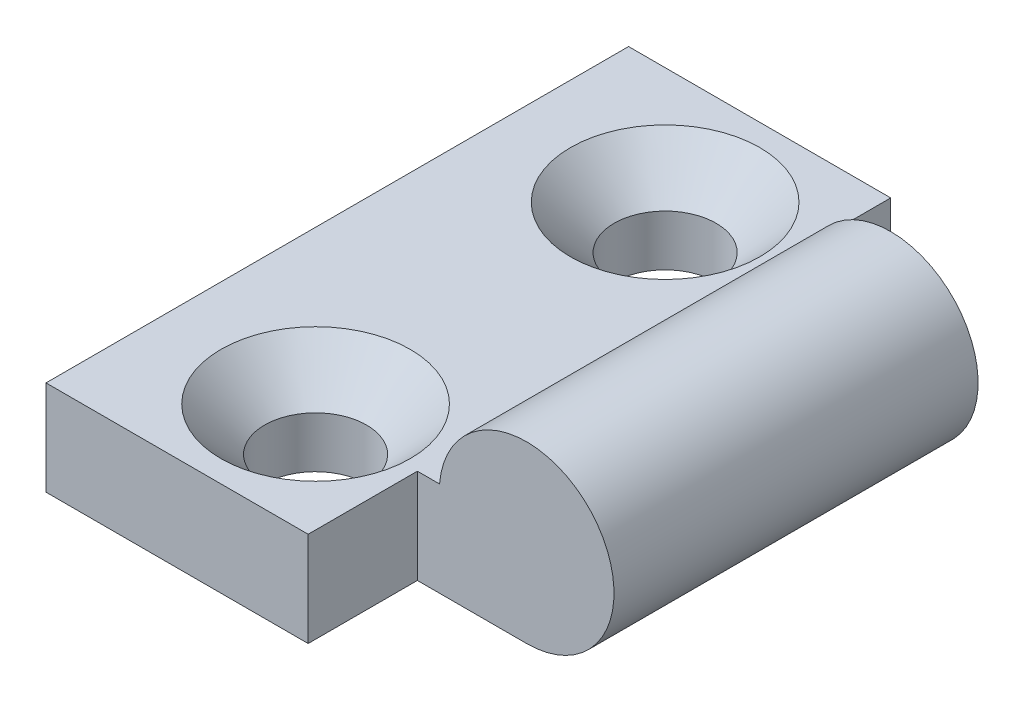
from build123d import *

# Parameters (mm, degrees)
SKETCH_1_W          = 25.5
SKETCH_1_H          = 40
EXTRUDE_1_DEPTH     = 6.5
SKETCH_2_R          = 6
EXTRUDE_2_DEPTH     = 40
SKETCH_3_W          = 13.5
SKETCH_3_H          = 7.5
CUT_EXTRUDE_1_DEPTH = 30.925950277
SKETCH_5_R          = 3.5
CUT_EXTRUDE_2_DEPTH = 29.174678348
CHAMFER_1_SIZE      = 3


with BuildPart() as part:
    # 草图1 → 凸台-拉伸1 (new body)
    with BuildSketch(Plane(origin=(0, 0, 0), x_dir=(1, 0, 0), z_dir=(0, 1, 0))):
        Rectangle(SKETCH_1_W, SKETCH_1_H)
    extrude(amount=EXTRUDE_1_DEPTH)

    # 草图2 → 凸台-拉伸2 (add)
    with BuildSketch(Plane.XY.offset(20)):
        with Locations((12.75, 6)):
            Circle(SKETCH_2_R)
    extrude(amount=-EXTRUDE_2_DEPTH)

    # 草图3 → 切除-拉伸1 (cut, through all)
    with BuildSketch(Plane.XZ):
        with Locations((12, 16.25)):
            Rectangle(SKETCH_3_W, SKETCH_3_H)
        with Locations((12, -16.25)):
            Rectangle(SKETCH_3_W, SKETCH_3_H)
    extrude(amount=-CUT_EXTRUDE_1_DEPTH, mode=Mode.SUBTRACT)

    # 草图5 → 切除-拉伸2 (cut, through all)
    with BuildSketch(Plane(origin=(0, 6.5, 0), x_dir=(1, 0, 0), z_dir=(0, 1, 0))):
        with Locations(Location((-2.239565186, 12, 0), (0, 0, 270))):
            Circle(SKETCH_5_R)
        with Locations(Location((-2.239565186, -12, 0), (0, 0, 270))):
            Circle(SKETCH_5_R)
    extrude(amount=-CUT_EXTRUDE_2_DEPTH, mode=Mode.SUBTRACT)

    # 倒角1
    chamfer_1_edges = [part.edges().sort_by_distance(p)[0] for p in [
        (-2.239565186, 6.5, -15.5),
        (-2.239565186, 6.5, 8.5),
    ]]
    chamfer(chamfer_1_edges, length=CHAMFER_1_SIZE)


solid = part.part
